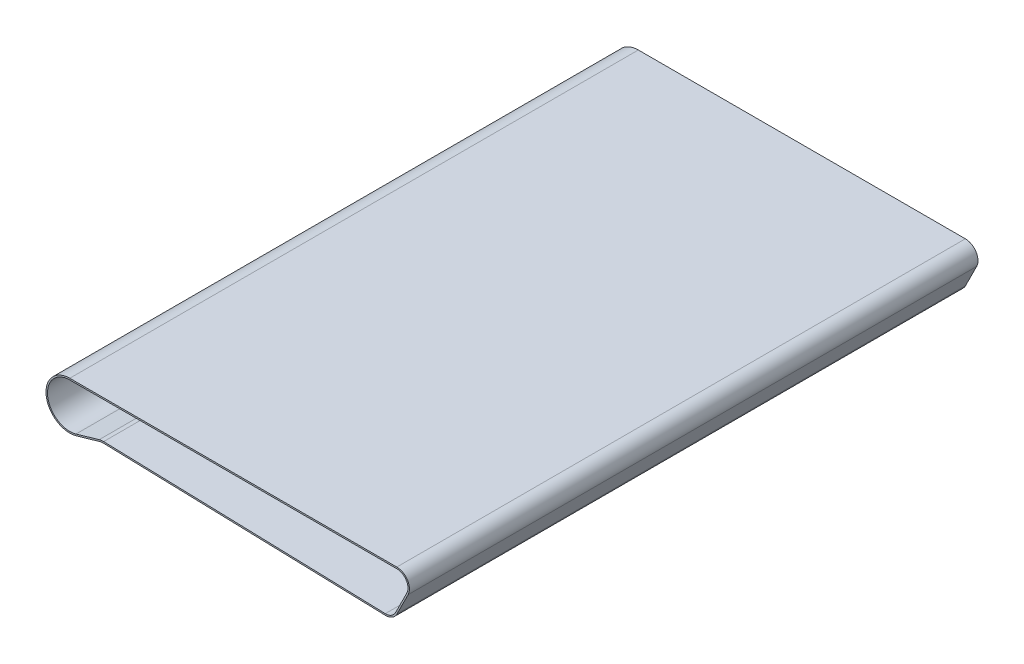
from build123d import *

# Parameters (mm, degrees)
EXTRUDE_1_DEPTH = 382.5


with BuildPart() as part:
    # 草图1 → 凸台-拉伸1 (new, symmetric)
    with BuildSketch(Plane.XY):
        with BuildLine():
            Line((8.903211102, -30.736506504), (40.131056429, -21.690973006))
            ThreePointArc((40.131056429, -21.690973006), (42.792421792, -21.139798433), (45.507033287, -21.007346764))
            Line((45.507033287, -21.007346764), (424.507453379, -31.992863144))
            ThreePointArc((424.507453379, -31.992863144), (433.726976259, -29.589033052), (440.205262247, -22.602631123))
            Line((440.205262247, -22.602631123), (455.205262247, 7.397368877))
            ThreePointArc((455.205262247, 7.397368877), (454.461063742, 23.937428906), (440, 32))
            Line((440, 32), (0, 32))
            ThreePointArc((0, 32), (-31.682552045, -4.496209063), (8.903211102, -30.736506504))
        make_face()
        with BuildLine():
            Line((0, 30), (440, 30))
            ThreePointArc((440, 30), (452.759762125, 22.885966682), (453.416407865, 8.291796068))
            Line((453.416407865, 8.291796068), (438.416407865, -21.708203932))
            ThreePointArc((438.416407865, -21.708203932), (432.700273169, -27.872676222), (424.56540004, -29.993702774))
            Line((424.56540004, -29.993702774), (45.564979948, -19.008186394))
            ThreePointArc((45.564979948, -19.008186394), (42.54012714, -19.155775396), (39.574605735, -19.769941349))
            Line((39.574605735, -19.769941349), (8.346760408, -28.815474848))
            ThreePointArc((8.346760408, -28.815474848), (-29.702392542, -4.215195996), (0, 30))
        make_face(mode=Mode.SUBTRACT)
    extrude(amount=EXTRUDE_1_DEPTH, both=True)


solid = part.part
